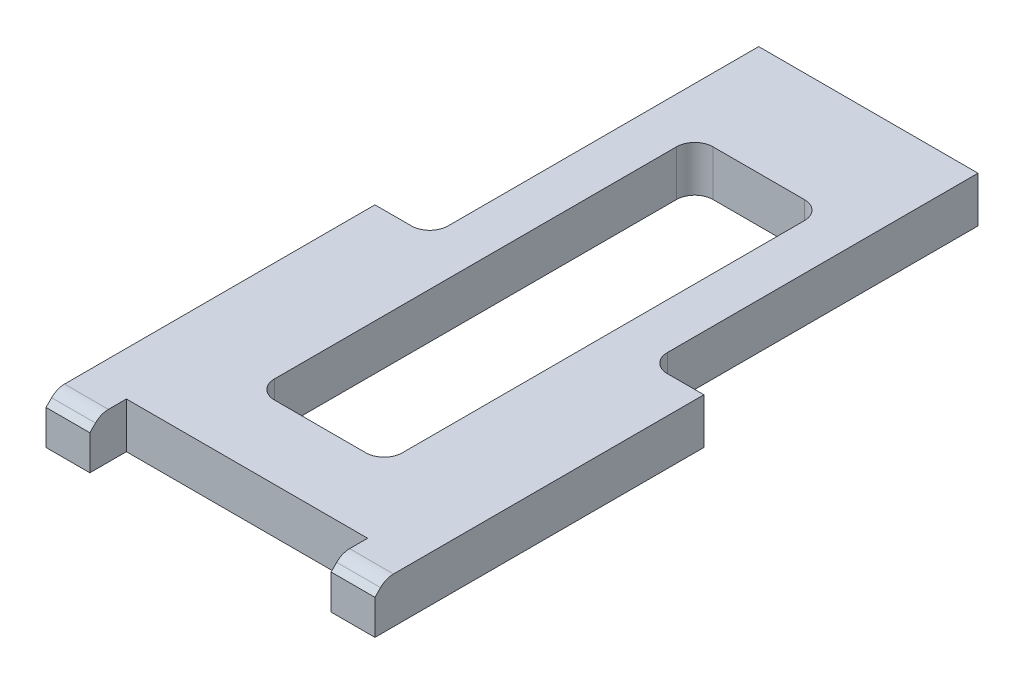
from build123d import *

# Parameters (mm, degrees)
SKETCH1_W           = 90
SKETCH1_H           = 12.5
BOSS_EXTRUDE1_DEPTH = 180
SKETCH2_W           = 66
SKETCH2_H           = 10
CUT_EXTRUDE1_DEPTH  = 186.960345235
CHAMFER1_SIZE       = 3
FILLET1_R           = 5
SKETCH3_W           = 15
SKETCH3_H           = 90
CUT_EXTRUDE2_DEPTH  = 186.960345235
SKETCH4_W           = 35
SKETCH4_H           = 120
CUT_EXTRUDE3_DEPTH  = 186.960345235
FILLET2_R           = 5
FILLET3_R           = 5


with BuildPart() as part:
    # Sketch1 → Boss-Extrude1 (new body)
    with BuildSketch(Plane.XY):
        Rectangle(SKETCH1_W, SKETCH1_H)
    extrude(amount=BOSS_EXTRUDE1_DEPTH)

    # Sketch2 → Cut-Extrude1 (cut, through all)
    with BuildSketch(Plane(origin=(0, 6.25, 0), x_dir=(1, 0, 0), z_dir=(0, 1, 0))):
        with Locations((0, -175)):
            Rectangle(SKETCH2_W, SKETCH2_H)
    extrude(amount=-CUT_EXTRUDE1_DEPTH, mode=Mode.SUBTRACT)

    # Chamfer1
    chamfer1_edges = [part.edges().sort_by_distance(p)[0] for p in [
        (39, 6.25, 180),
        (-39, 6.25, 180),
    ]]
    chamfer(chamfer1_edges, length=CHAMFER1_SIZE)

    # Fillet1
    fillet1_edges = [part.edges().sort_by_distance(p)[0] for p in [
        (39, 6.25, 177),
        (-39, 6.25, 177),
    ]]
    fillet(fillet1_edges, radius=FILLET1_R)

    # Sketch3 → Cut-Extrude2 (cut, through all)
    with BuildSketch(Plane(origin=(0, 6.25, 0), x_dir=(1, 0, 0), z_dir=(0, 1, 0))):
        with Locations((37.5, -45)):
            Rectangle(SKETCH3_W, SKETCH3_H)
        with Locations((-37.5, -45)):
            Rectangle(SKETCH3_W, SKETCH3_H)
    extrude(amount=-CUT_EXTRUDE2_DEPTH, mode=Mode.SUBTRACT)

    # Sketch4 → Cut-Extrude3 (cut, through all)
    with BuildSketch(Plane(origin=(0, 6.25, 0), x_dir=(1, 0, 0), z_dir=(0, 1, 0))):
        with Locations((0, -90)):
            Rectangle(SKETCH4_W, SKETCH4_H)
    extrude(amount=-CUT_EXTRUDE3_DEPTH, mode=Mode.SUBTRACT)

    # Fillet2
    fillet2_edges = [part.edges().sort_by_distance(p)[0] for p in [
        (-17.5, 0, 150),
        (-17.5, 0, 30),
        (17.5, 0, 30),
        (17.5, 0, 150),
    ]]
    fillet(fillet2_edges, radius=FILLET2_R)

    # Fillet3
    fillet3_edges = [part.edges().sort_by_distance(p)[0] for p in [
        (30, 0, 90),
        (-30, 0, 90),
    ]]
    fillet(fillet3_edges, radius=FILLET3_R)


solid = part.part
